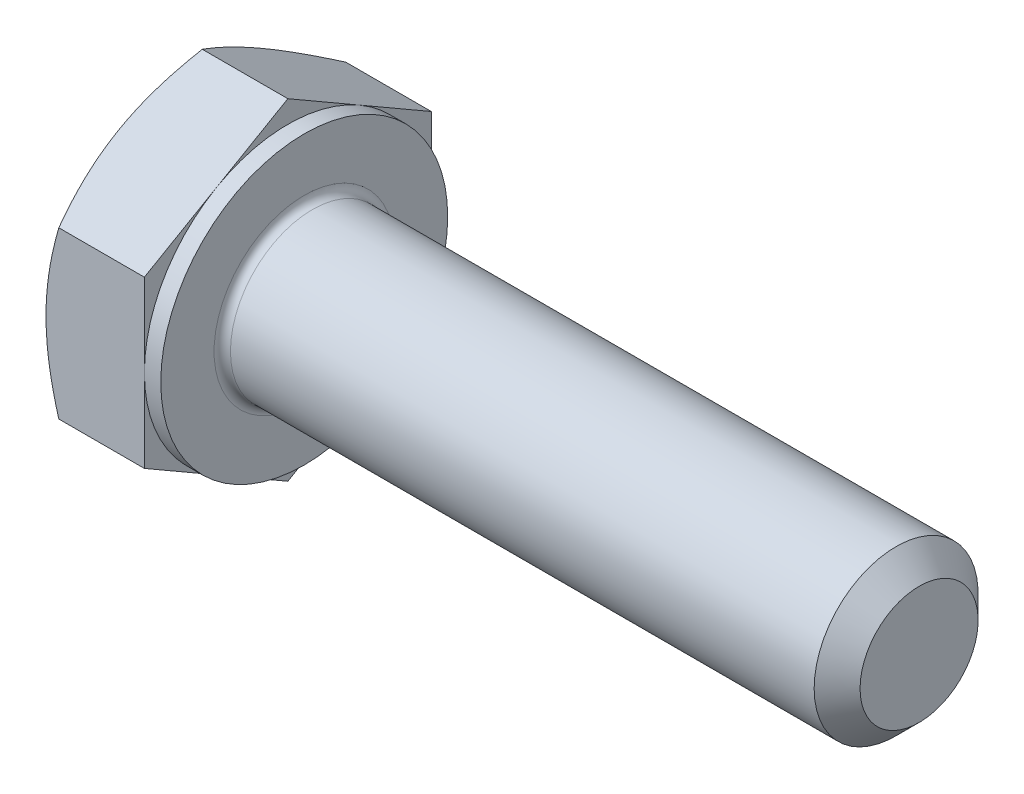
SolidWorks part; units mm, degrees
extrude "基体-拉伸" add sketch "草图1" along normal blind 2.8
sketch "草图1" plane through (0, 0, 0) normal (1, 0, 0) x (0, 0, -1)
  line L0 (3.5, 2.0207) -> (3.5, -2.0207)
  line L1 (-3.5, 2.0207) -> (-3.5, -2.0207)
  line L2 (3.5, -2.0207) -> (0, -4.0415)
  line L3 (0, -4.0415) -> (-3.5, -2.0207)
  line L4 (3.5, 2.0207) -> (0, 4.0415)
  line L5 (0, 4.0415) -> (-3.5, 2.0207)
revolve "切除-旋转1" cut sketch "草图3" angle 360 about L6
sketch "草图3" plane through (0, 0, 0) normal (0, 0, 1) x (1, 0, 0)
  line L0 (0, 3.5) -> (3.1994, 9.0415)
  line L1 (0, 4.0415) -> (0, 2.0207) construction
  line L2 (3.1994, 9.0415) -> (3.1994, 14.0415)
  line L3 (3.1994, 14.0415) -> (-10, 14.0415)
  line L4 (-10, 14.0415) -> (-10, 3.5)
  line L5 (-10, 3.5) -> (0, 3.5)
  line L6 (0, 0) -> (99.06, 0) construction
  line L7 (2.8, 4.0415) -> (0, 4.0415) construction
revolve "凸台-旋转1" add sketch "草图2" angle 360 about L7
sketch "草图2" plane through (0, 0, 0) normal (0, 0, 1) x (1, 0, 0)
  line L0 (0, 2.0207) -> (0, -2.0207) construction
  line L1 (0, 0) -> (17.8, 0)
  line L2 (0, 0) -> (0, 2)
  line L3 (0, 2) -> (17.8, 2)
  line L4 (17.8, 0) -> (17.8, 1.3938)
  line L5 (2.8, 4.0415) -> (2.8, 2.0207) construction
  line L7 (0, 0) -> (96.52, 0) construction
  line L8 (17.8, -1.3938) -> (90.335, -2) construction
  line L9 (0, -2) -> (90.335, -2) construction
  line L10 (3.5, 15.24) -> (3.5, -1.27) construction
  line L11 (2.8, 15.24) -> (2.8, -1.27) construction
  line L12 (2.8, 2.0207) -> (2.8, -2.0207) construction
  line L14 (17.8, 2) -> (17.8, 1.3938)
  dimension "l" = 15
  dimension "m" = 4
  dimension "Minor_dia" = 2.7876
  dimension "p" = 0.7
  dimension "h" = 15
cosmetic thread "螺旋线1" parameters "Thread_length"=14.3, "Thread_minor"=2.7876
material "不锈钢"
ref_plane "前视" through (0, 0, 0) normal (0, 0, 1) x (1, 0, 0)
ref_plane "上视" through (0, 0, 0) normal (0, 1, 0) x (1, 0, 0)
ref_plane "右视" through (0, 0, 0) normal (1, 0, 0) x (0, 0, -1)
sketch "草图5" plane through (0, 0, 0) normal (0, 0, 1) x (1, 0, 0)
  line L0 (2.8, 3.5) -> (-0.3994, 9.0415)
  line L1 (2.8, 4.0415) -> (2.8, 2.0207) construction
  line L2 (-0.3994, 9.0415) -> (-0.3994, 14.0415)
  line L3 (-0.3994, 14.0415) -> (9.6006, 14.0415)
  line L4 (9.6006, 14.0415) -> (9.6006, 3.5)
  line L5 (9.6006, 3.5) -> (2.8, 3.5)
  line L7 (2.8, 4.0415) -> (0.3126, 4.0415) construction
  line L8 (0, 0) -> (99.06, 0) construction
  line L9 (0, 0) -> (99.06, 0) construction
revolve "切除-旋转2" cut sketch "草图5" angle 360 about L8
sketch "草图4" plane through (0, 0, 0) normal (0, 0, 1) x (1, 0, 0)
  line L1 (2.8, 4.0415) -> (2.8, 2.0207) construction
  line L2 (2.8, 3.5) -> (2.4, 3.5)
  line L3 (2.8, 3.5) -> (2.8, 14.0415)
  line L4 (2.8, 14.0415) -> (2.4, 14.0415)
  line L5 (0, 0) -> (95.25, 0) construction
  line L6 (0, 0) -> (96.52, 0) construction
  line L7 (2.4, 3.5) -> (2.4, 14.0415)
  line L8 (2.4874, 4.0415) -> (0.3126, 4.0415) construction
revolve "切除-旋转3" cut sketch "草图4" angle 360 about L5
chamfer "倒角" distance 0.56 angle 45 1 edges at (17.8, 0, 2)
fillet "圆角" radius 0.2 1 edges at (2.8, 0, -2)
sketch "草图6" plane through (0, 0, 0) normal (0, 0, 1) x (1, 0, 0)
  line L0 (3.35, -1.3938) -> (3, -2)
  line L1 (3.35, -1.3938) -> (3.7, -2)
  line L2 (3.7, -2) -> (3.7, -2.5)
  line L3 (-3.175, 0) -> (5.1513, 0) construction
  line L5 (3.7, -2.5) -> (3, -2.5)
  line L6 (3, -2.5) -> (3, -2)
  arc A0 (3, -2) -> (2.8, -2.2) centre (3, -2.2) ccw construction
revolve "切除-旋转4" [suppressed] cut sketch "草图6" angle 360 about L3
pattern_linear "阵列(线性)1" [suppressed]
equation "\"D3@草图1\" = \"s@草图1\" / 2"
equation "\"D4@草图1\" = \"D3@草图1\""
equation "\"D5@草图1\" = \"D4@草图1\""
equation "\"D1@草图3\" = \"s@草图1\" / 2"
equation "\"D1@草图5\" = \"s@草图1\" / 2"
equation "\"Head_ch_ang@草图5\" = \"Head_ch_ang@草图3\""
equation "\"D1@草图4\" = \"s@草图1\""
equation "\"Diameter@草图6\" = \"m@草图2\""
equation "\"Overcut@草图6\" = \"m@草图2\" * 1.25"
equation "\"Minor_dia@草图2\" = \"m@草图2\"-\"p@草图2\" * 1.732"
equation "\"Thread_minor@螺旋线1\" = \"Minor_dia@草图2\""
equation "\"Thread_minor@草图6\" = \"Minor_dia@草图2\""
equation "\"D1@倒角\" = \"p@草图2\"*0.8"
equation "\"Thread_length@螺旋线1\" = \"l@草图2\" - \"p@草图2\""
equation "\"Num_threads@阵列(线性)1\" = \"l@草图2\" / \"p@草图2\""
